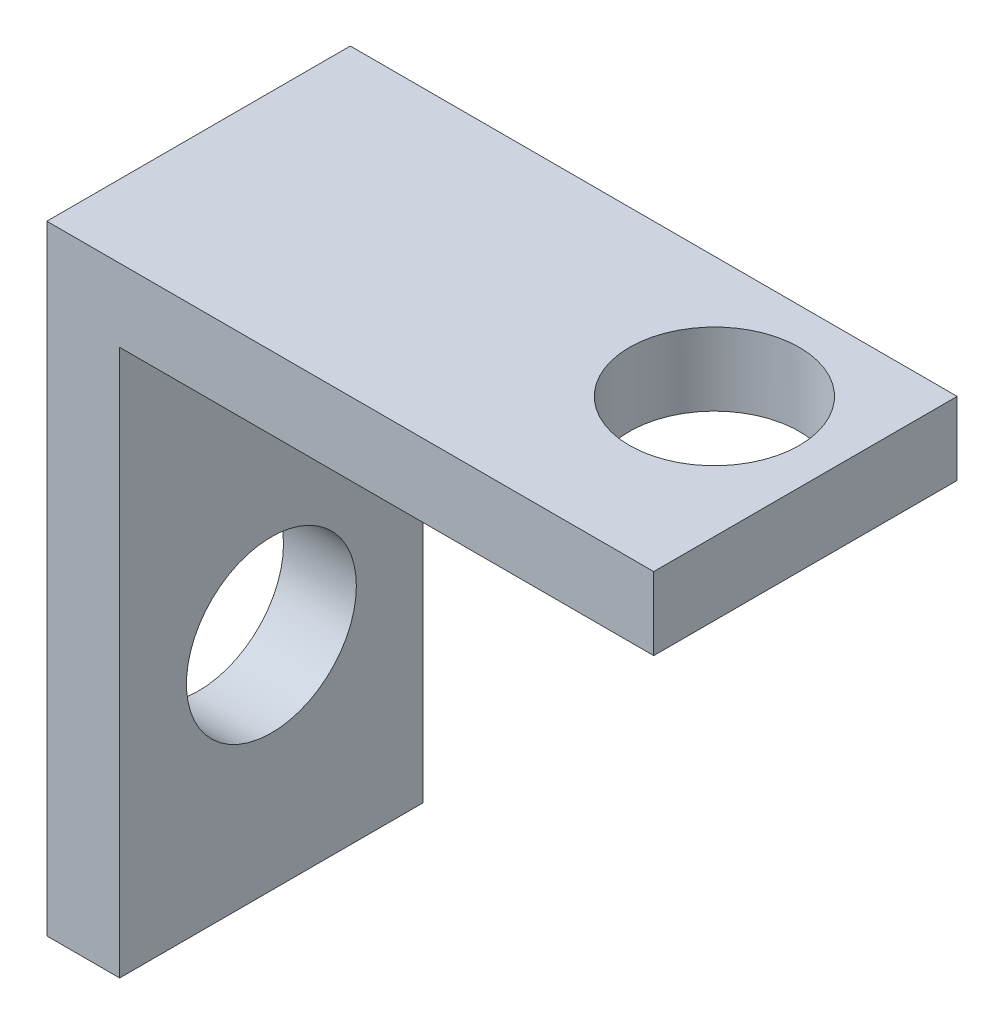
SolidWorks part; units mm, degrees
ref_plane "Front Plane" through (0, 0, 0) normal (0, 0, 1) x (1, 0, 0)
ref_plane "Top Plane" through (0, 0, 0) normal (0, 1, 0) x (1, 0, 0)
ref_plane "Right Plane" through (0, 0, 0) normal (1, 0, 0) x (0, 0, -1)
other "Configuration Table"
sketch "Sketch1" plane through (0, 0, 0) normal (0, 1, 0) x (1, 0, 0)
  line L1 (-20, -25) -> (20, -25)
  line L2 (-20, -25) -> (-20, 25)
  line L3 (-20, 25) -> (20, 25)
  line L4 (20, -25) -> (20, 25)
  line L5 (-20, -25) -> (20, 25) construction
  line L6 (-20, 25) -> (20, -25) construction
  point P0 (0, 0)
  dimension "D1" = 40
  dimension "D2" = 50
extrude "Boss-Extrude1" add sketch "Sketch1" along normal blind 12
sketch "Sketch2" plane through (0, 12, 0) normal (0, 1, 0) x (1, 0, 0)
  line L0 (0, 25) -> (0, 0) construction
  line L1 (20, 25) -> (-20, 25) construction
  circle A0 centre (0, 5) radius 14
  dimension "D1" = 28
  dimension "D2" = 20
extrude "Cut-Extrude1" cut sketch "Sketch2" against normal through all both and the other way through all
other "Move Face2" face at (-20, 6, 0) parameters "D1"=60
sketch "Sketch3" plane through (0, 0, 0) normal (0, 1, 0) x (1, 0, 0)
  line L0 (-80, -25) -> (20, -25) construction
  line L1 (-80, 25) -> (-68, 25)
  line L2 (-80, 25) -> (-80, -25)
  line L3 (-80, -25) -> (-68, -25)
  line L4 (-68, 25) -> (-68, -25)
  dimension "D1" = 12
extrude "Boss-Extrude2" add sketch "Sketch3" against normal blind 90
sketch "Sketch4" plane through (-68, 0, 0) normal (1, 0, 0) x (0, 0, -1)
  line L0 (-25, -90) -> (25, -90) construction
  circle A0 centre (0, -53.54) radius 14
  dimension "D1" = 28
  dimension "D2" = 36.46
extrude "Cut-Extrude2" cut sketch "Sketch4" against normal through all both and the other way through all
